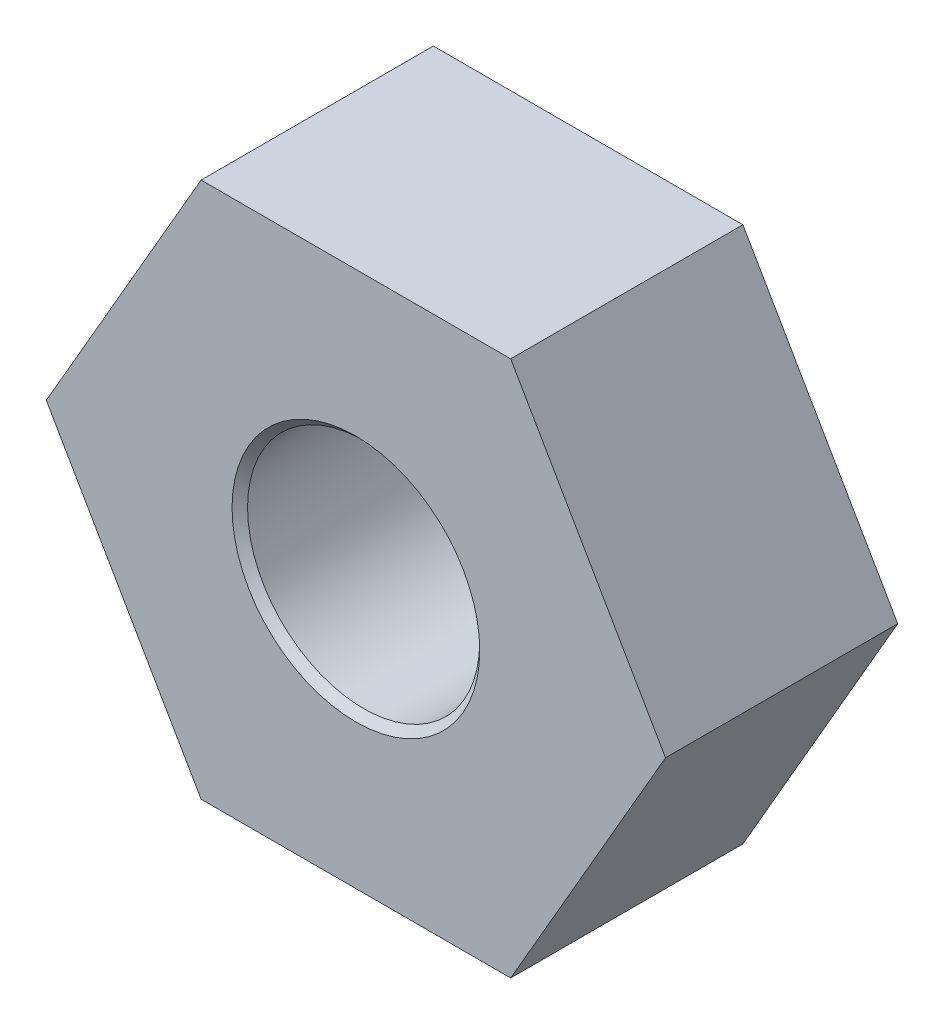
SolidWorks part; units mm, degrees
ref_plane "Front Plane" through (0, 0, 0) normal (0, 0, 1) x (1, 0, 0)
ref_plane "Top Plane" through (0, 0, 0) normal (0, 1, 0) x (1, 0, 0)
ref_plane "Right Plane" through (0, 0, 0) normal (1, 0, 0) x (0, 0, -1)
other "Configuration Table"
sketch "Sketch1" plane through (0, 0, 0) normal (0, 0, 1) x (1, 0, 0)
  line L1 (2, -3.4641) -> (4, 0)
  line L2 (4, 0) -> (2, 3.4641)
  line L3 (2, 3.4641) -> (-2, 3.4641)
  line L4 (-2, 3.4641) -> (-4, 0)
  line L5 (-4, 0) -> (-2, -3.4641)
  line L6 (-2, -3.4641) -> (2, -3.4641)
  circle A0 centre (0, 0) radius 1.5
  circle A1 centre (0, 0) radius 3.4641 construction
  point P3 (0, 3.4641)
  dimension "D1" = 3
  dimension "D2" = 4
extrude "Boss-Extrude1" add sketch "Sketch1" along normal blind 3
chamfer "Chamfer1" distance 0.1 angle 45 2 edges at (1.5, 0, 0) (1.5, 0, 3)
